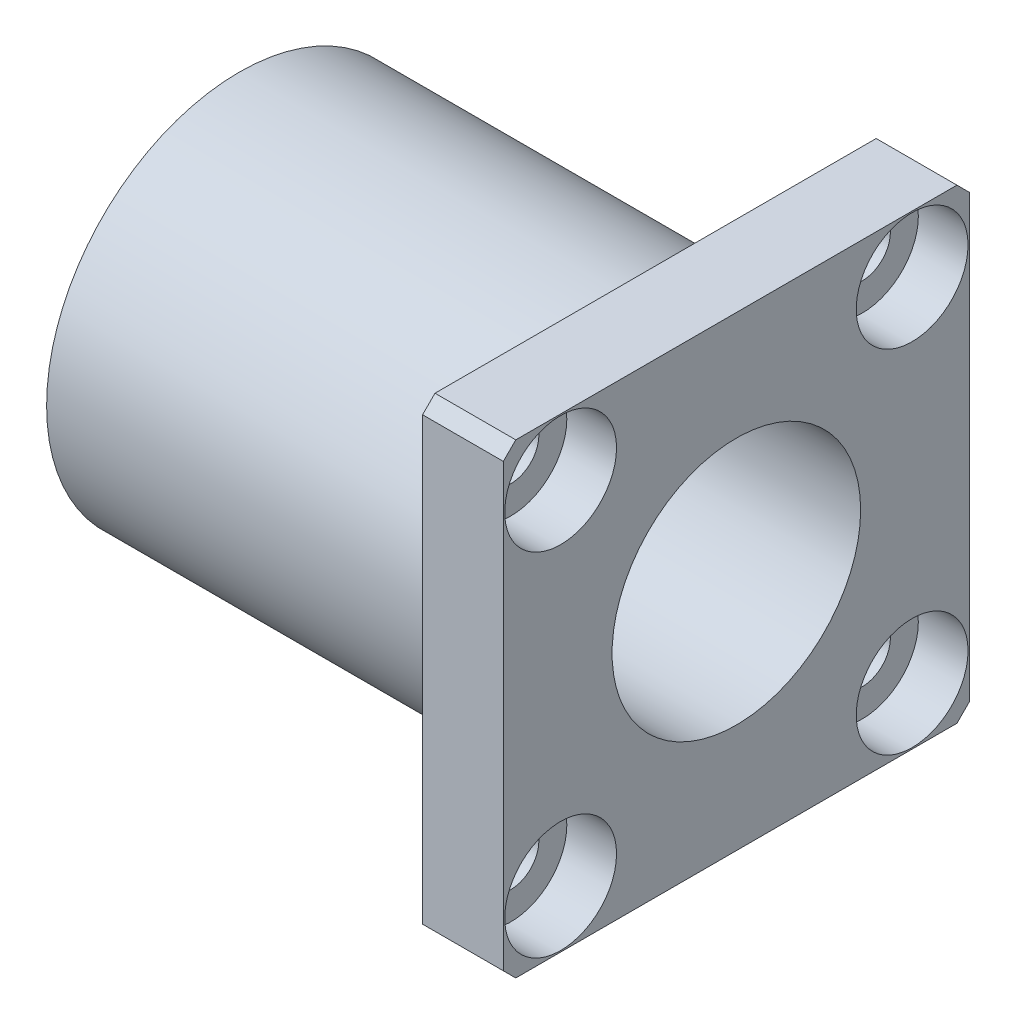
SolidWorks part; units mm, degrees
ref_plane "Front Plane" through (0, 0, 0) normal (0, 0, 1) x (1, 0, 0)
ref_plane "Top Plane" through (0, 0, 0) normal (0, 1, 0) x (1, 0, 0)
ref_plane "Right Plane" through (0, 0, 0) normal (1, 0, 0) x (0, 0, -1)
sketch "Sketch1" plane through (0, 0, 0) normal (1, 0, 0) x (0, 0, -1)
  circle A0 centre (0, 0) radius 31
  circle A1 centre (0, 0) radius 20
  dimension "D1" = 40
  dimension "D2" = 62
extrude "Boss-Extrude1" add sketch "Sketch1" along normal blind 67
sketch "Sketch2" plane through (67, 0, 0) normal (1, 0, 0) x (0, 0, -1)
  line L1 (-37.5, 37.5) -> (37.5, 37.5)
  line L2 (-37.5, 37.5) -> (-37.5, -37.5)
  line L3 (-37.5, -37.5) -> (37.5, -37.5)
  line L4 (37.5, 37.5) -> (37.5, -37.5)
  line L5 (-37.5, 37.5) -> (37.5, -37.5) construction
  line L6 (-37.5, -37.5) -> (37.5, 37.5) construction
  circle A0 centre (0, 0) radius 20
  dimension "D1" = 75
  dimension "D2" = 75
extrude "Boss-Extrude2" add sketch "Sketch2" along normal blind 13
hole_wizard "CBORE for M8 Hex Head Bolt1" positions "Sketch3" profile "Sketch4" counterbore size "M8" standard "GB" end condition through all
sketch "Sketch3" plane through (80, 0, 0) normal (1, 0, 0) x (0, 0, -1)
  line L0 (0, 0) -> (0, 40) construction
  line L2 (0, 0) -> (28.2843, 28.2843) construction
  circle A0 centre (0, 0) radius 40 construction
  point P6 (28.2843, 28.2843)
  point P30 (28.2843, -28.2843)
  point P31 (-28.2843, -28.2843)
  point P32 (-28.2843, 28.2843)
  dimension "D2" = 4
  dimension "D1" = 45
sketch "Sketch4" plane through (80, 28.2843, -28.2843) normal (0, 1, 0) x (0, 0, -1)
  line L0 (0, 0) -> (0, 80)
  line L1 (0, 80) -> (4.5, 80)
  line L3 (4.5, 80) -> (4.5, 8)
  line L4 (4.5, 8) -> (9, 8)
  line L5 (9, 8) -> (9, 0)
  line L7 (9, 0) -> (0, 0)
  line L11 (0, -6.35) -> (0, 107.95) construction
  dimension "通孔孔直径" = 9
  dimension "通孔孔深度" = 80
  dimension "柱形沉头孔直径" = 18
  dimension "柱形沉头孔深度" = 8
chamfer "Chamfer1" distance 2 angle 45 4 edges at (73.5, 37.5, 37.5) (73.5, 37.5, -37.5) (73.5, -37.5, -37.5) (73.5, -37.5, 37.5)
